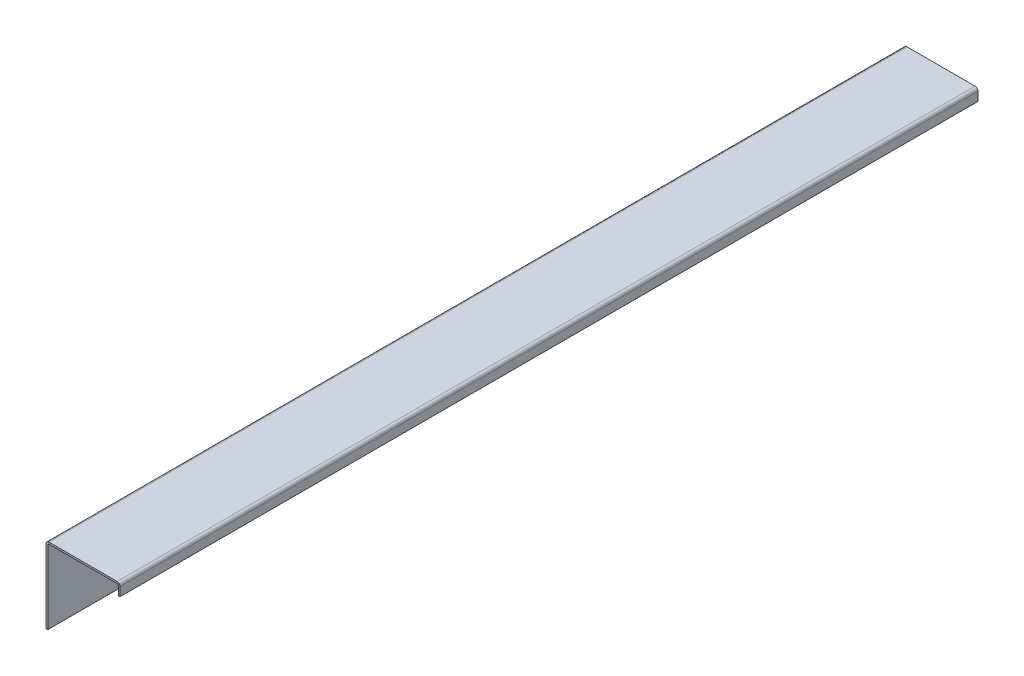
SolidWorks part; units mm, degrees
material "1023 Carbon Steel Plate (SS)"
ref_plane "Front Plane" through (0, 0, 0) normal (0, 0, 1) x (1, 0, 0)
ref_plane "Top Plane" through (0, 0, 0) normal (0, 1, 0) x (1, 0, 0)
ref_plane "Right Plane" through (0, 0, 0) normal (1, 0, 0) x (0, 0, -1)
sketch "Sketch1" plane through (0, 0, 0) normal (0, 0, 1) x (1, 0, 0)
  line L0 (0, 0) -> (0, 125)
  line L1 (5, 130) -> (121, 130)
  line L2 (126, 125) -> (126, 110)
  line L3 (3, 0) -> (3, 125)
  line L4 (5, 127) -> (121, 127)
  line L5 (123, 125) -> (123, 110)
  line L6 (126, 110) -> (123, 110)
  line L7 (0, 0) -> (3, 0)
  arc A0 (121, 130) -> (126, 125) centre (121, 125) cw
  arc A1 (0, 125) -> (5, 130) centre (5, 125) cw
  arc A2 (3, 125) -> (5, 127) centre (5, 125) cw
  arc A3 (121, 127) -> (123, 125) centre (121, 125) cw
  point P7 (126, 130)
  point P10 (0, 130)
  dimension "D4" = 5
  dimension "D1" = 130
  dimension "D2" = 126
  dimension "D3" = 20
  dimension "D5" = 3
extrude "Boss-Extrude1" add sketch "Sketch1" along normal blind 1460 contours L7 L3 A2 L4 A3 L5 L6 L2 A0 L1 A1 L0
sketch "Sketch2" plane through (0, 0, 0) normal (-1, 0, 0) x (0, 0, 1)
  line L0 (1460, 0) -> (0, 0) construction
  line L1 (0, 0) -> (0, 125) construction
  circle A0 centre (121, 80) radius 4
  circle A1 centre (1339, 80) radius 4
  circle A2 centre (933, 80) radius 4
  circle A3 centre (527, 80) radius 4
  circle A4 centre (121, 20) radius 4
  circle A5 centre (1339, 20) radius 4
  circle A6 centre (933, 20) radius 4
  circle A7 centre (527, 20) radius 4
  dimension "D7" = 8
  dimension "D1" = 60
  dimension "D2" = 20
  dimension "D3" = 406
  dimension "D4" = 121
  dimension "D5" = 406
  dimension "D6" = 406
extrude "Cut-Extrude1" cut sketch "Sketch2" against normal blind 1460
